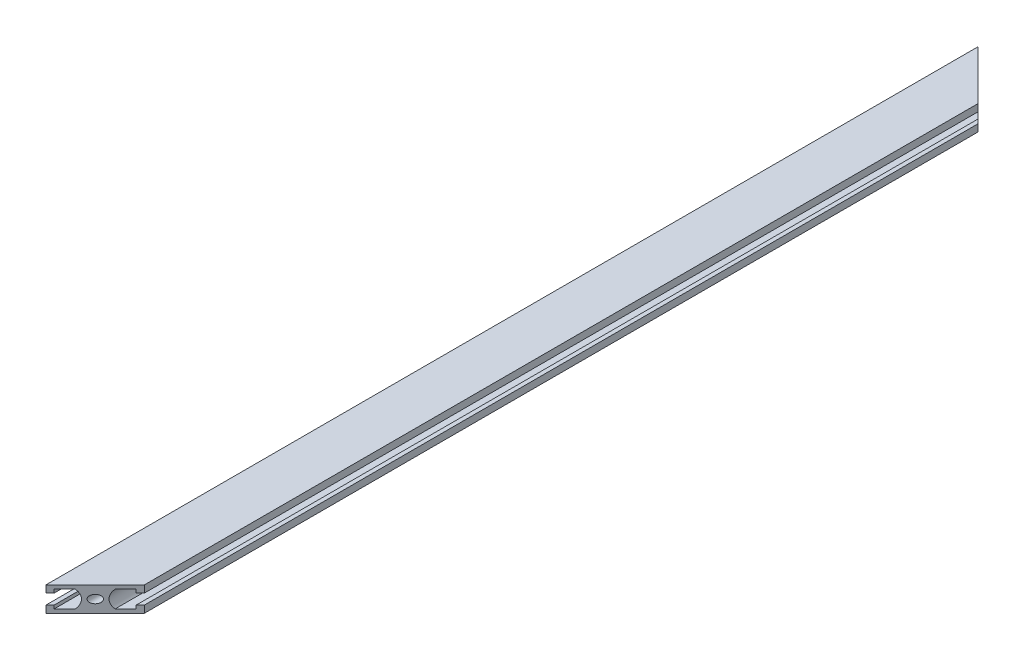
from build123d import *

# Parameters (mm, degrees)
MODEL_R                = 2.5
EXTRUDE_1_DEPTH        = 284
CUT_EXTRUDE_1_DEPTH    = 2410.767812852
HOLE_WIZARD_M4_1_D     = 3.3
HOLE_WIZARD_M4_1_DEPTH = 11.5
HOLE_WIZARD_M4_1_TIP   = 0.991420021


with BuildPart() as part:
    # Model → 凸台-拉伸1 (new, symmetric)
    with BuildSketch(Plane.XY):
        with BuildLine():
            Line((2390.427059452, 419.756797217), (2392.927059452, 419.756797217))
            Line((2392.927059452, 419.756797217), (2392.927059452, 415.406797217))
            Line((2392.927059452, 415.406797217), (2362.927059452, 415.406797217))
            Line((2362.927059452, 415.406797217), (2362.927059452, 419.756797217))
            Line((2362.927059452, 419.756797217), (2365.427059452, 419.756797217))
            Line((2365.427059452, 419.756797217), (2365.427059452, 417.706797217))
            Line((2365.427059452, 417.706797217), (2371.857059452, 417.706797217))
            ThreePointArc((2371.857059452, 417.706797217), (2373.727059452, 422.906797217), (2371.857059452, 428.106797217))
            Line((2371.857059452, 428.106797217), (2365.427059452, 428.106797217))
            Line((2365.427059452, 428.106797217), (2365.427059452, 426.056797217))
            Line((2365.427059452, 426.056797217), (2362.927059452, 426.056797217))
            Line((2362.927059452, 426.056797217), (2362.927059452, 430.406797217))
            Line((2362.927059452, 430.406797217), (2392.927059452, 430.406797217))
            Line((2392.927059452, 430.406797217), (2392.927059452, 426.056797217))
            Line((2392.927059452, 426.056797217), (2390.427059452, 426.056797217))
            Line((2390.427059452, 426.056797217), (2390.427059452, 428.106797217))
            Line((2390.427059452, 428.106797217), (2383.994799144, 428.106797217))
            ThreePointArc((2383.994799144, 428.106797217), (2382.127059452, 422.906797217), (2383.994799144, 417.706797217))
            Line((2383.994799144, 417.706797217), (2390.427059452, 417.706797217))
            Line((2390.427059452, 417.706797217), (2390.427059452, 419.756797217))
        make_face()
        with Locations((2377.927059452, 422.906797217)):
            Circle(MODEL_R, mode=Mode.SUBTRACT)
    extrude(amount=EXTRUDE_1_DEPTH, both=True)

    # 草图1 → 切除-拉伸1 (cut, through all)
    with BuildSketch(Plane(origin=(0, 430.406797217, 0), x_dir=(1, 0, 0), z_dir=(0, 1, 0))):
        Polygon((2362.927059452, 284), (2392.927059452, 254), (2392.927059452, 284), align=None)
        Polygon((2362.927059452, -284), (2392.927059452, -254), (2392.927059452, -284), align=None)
    extrude(amount=-CUT_EXTRUDE_1_DEPTH, mode=Mode.SUBTRACT)

    # M4 螺纹孔1
    with Locations(Plane(origin=(0, 415.406797217, 0), x_dir=(-1, 0, 0), z_dir=(0, -1, 0))):
        with Locations((-2377.927059452, -219), (-2377.927059452, -191), (-2377.927059452, 191), (-2377.927059452, 219)):
            Hole(HOLE_WIZARD_M4_1_D / 2, depth=HOLE_WIZARD_M4_1_DEPTH)
            with Locations((0, 0, -(HOLE_WIZARD_M4_1_DEPTH + HOLE_WIZARD_M4_1_TIP / 2))):  # 118° drill point
                Cone(0, HOLE_WIZARD_M4_1_D / 2, HOLE_WIZARD_M4_1_TIP, mode=Mode.SUBTRACT)


solid = part.part
